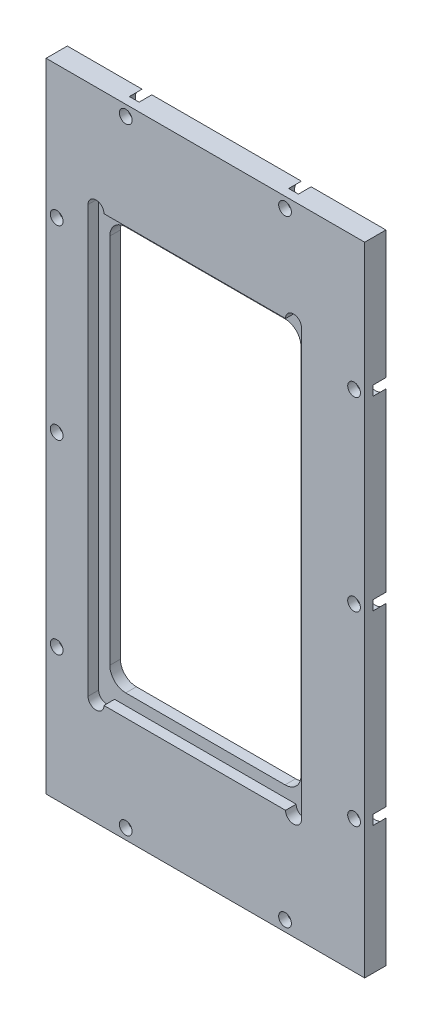
from build123d import *

# Parameters (mm, degrees)
SKETCH_1_W                   = 60
SKETCH_1_H                   = 120
EXTRUDE_1_DEPTH              = 2
SKETCH_2_W                   = 36
SKETCH_2_H                   = 76
CUT_EXTRUDE_1_DEPTH          = 68.201190466
SKETCH_3_W                   = 40.2
SKETCH_3_H                   = 80.2
CUT_EXTRUDE_2_DEPTH          = 2
HOLE_WIZARD_3_0_3_1_D        = 3
HOLE_WIZARD_3_0_3_1_DEPTH    = 2
FILLET_1_R                   = 3
HOLE_WIZARD_M2_1_D           = 2.4
HOLE_WIZARD_M2_1_CBORE_D     = 4.4
HOLE_WIZARD_M2_1_CBORE_DEPTH = 2.4


with BuildPart() as part:
    # 草图1 → 凸台-拉伸1 (new, symmetric)
    with BuildSketch(Plane.XY):
        Rectangle(SKETCH_1_W, SKETCH_1_H)
    extrude(amount=EXTRUDE_1_DEPTH, both=True)

    # 草图2 → 切除-拉伸1 (cut, through all)
    with BuildSketch(Plane.XY.offset(2)):
        with Locations((-2, 0)):
            Rectangle(SKETCH_2_W, SKETCH_2_H)
    extrude(amount=-CUT_EXTRUDE_1_DEPTH, mode=Mode.SUBTRACT)

    # 草图3 → 切除-拉伸2 (cut)
    with BuildSketch(Plane.XY.offset(2)):
        with Locations((-2, 0)):
            Rectangle(SKETCH_3_W, SKETCH_3_H)
    extrude(amount=-CUT_EXTRUDE_2_DEPTH, mode=Mode.SUBTRACT)

    # Ø3.0 (3) 直径孔1
    with Locations(Plane.XY.offset(2)):
        with Locations((-20.6, 40.1), (16.6, 40.1), (16.6, -40.1), (-20.6, -40.1)):
            Hole(HOLE_WIZARD_3_0_3_1_D / 2, depth=HOLE_WIZARD_3_0_3_1_DEPTH)

    # 圆角1
    fillet_1_edges = [part.edges().sort_by_distance(p)[0] for p in [
        (-20, -38, -1),
        (-20, 38, -1),
        (16, 38, -1),
        (16, -38, -1),
    ]]
    fillet(fillet_1_edges, radius=FILLET_1_R)

    # M2 六角凹头螺钉的柱形沉头孔1 (through all)
    with Locations(Plane(origin=(0, 0, -2), x_dir=(1, 0, 0), z_dir=(0, 0, -1))):
        with Locations((-28, 0), (28, 0), (-15, -58), (15, -58), (-28, -35), (28, -35), (-28, 35), (28, 35), (-15, 58), (15, 58)):
            CounterBoreHole(HOLE_WIZARD_M2_1_D / 2, HOLE_WIZARD_M2_1_CBORE_D / 2, HOLE_WIZARD_M2_1_CBORE_DEPTH)


solid = part.part
